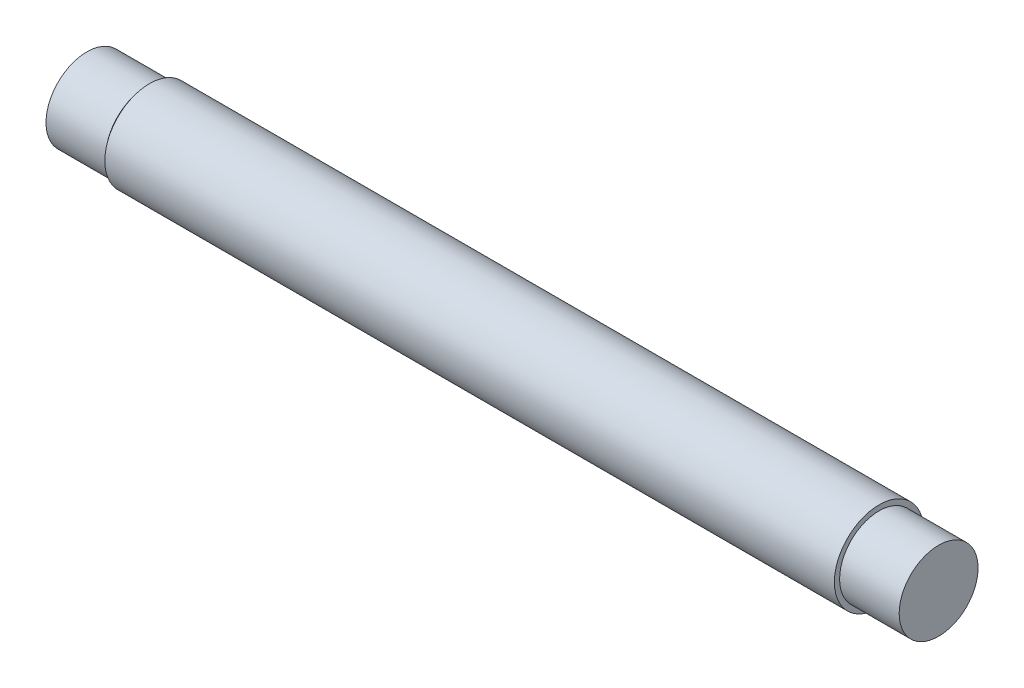
SolidWorks part; units mm, degrees
ref_plane "前视基准面" through (0, 0, 0) normal (0, 0, 1) x (1, 0, 0)
ref_plane "上视基准面" through (0, 0, 0) normal (0, 1, 0) x (1, 0, 0)
ref_plane "右视基准面" through (0, 0, 0) normal (1, 0, 0) x (0, 0, -1)
other "Configuration Table"
sketch "草图1" plane through (0, 0, 0) normal (0, 0, 1) x (1, 0, 0)
  line L0 (0, 0) -> (58.682, 0) construction
  line L1 (0, 0) -> (0, 27.5)
  line L2 (0, 27.5) -> (40, 27.5)
  line L3 (40, 27.5) -> (40, 26.5)
  line L4 (40, 26.5) -> (42, 26.5)
  line L5 (42, 26.5) -> (42, 30)
  line L6 (42, 30) -> (532, 30)
  line L7 (532, 30) -> (532, 26.5)
  line L8 (532, 26.5) -> (572, 26.5)
  line L9 (572, 26.5) -> (572, 0)
  line L10 (0, 0) -> (572, 0)
  dimension "D1" = 60
  dimension "D2" = 53
  dimension "D3" = 55
  dimension "D4" = 53
  dimension "D5" = 40
  dimension "D6" = 40
  dimension "D7" = 2
  dimension "D8" = 490
revolve "旋转1" add sketch "草图1" angle 360 about L0
